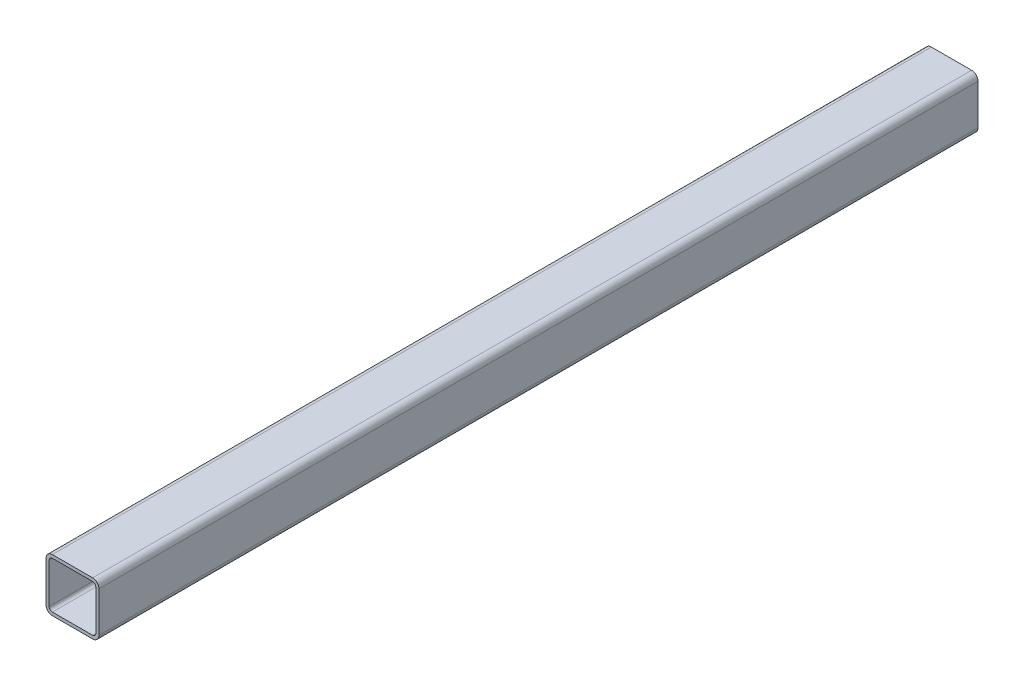
SolidWorks part; units mm, degrees
material "Q235B"
ref_plane "前视基准面" through (0, 0, 0) normal (0, 0, 1) x (1, 0, 0)
ref_plane "上视基准面" through (0, 0, 0) normal (0, 1, 0) x (1, 0, 0)
ref_plane "右视基准面" through (0, 0, 0) normal (1, 0, 0) x (0, 0, -1)
other "Configuration Table"
sketch "草图1" plane through (0, 0, 0) normal (1, 0, 0) x (0, 0, -1)
  line L0 (-415, 0) -> (415, 0)
other "Gb／6728-1986方形空心型钢 050 X 50 X 3(1)"
ref_plane "基准面1" through (0, 0, 415) normal (0, 0, -1) x (0, 1, 0)
sketch "Sketch1" plane through (0, 0, 415) normal (0, 0, -1) x (0, 1, 0)
  line L0 (-19, -22) -> (19, -22)
  line L1 (-22, -19) -> (-22, 19)
  line L2 (19, 22) -> (-19, 22)
  line L3 (22, 19) -> (22, -19)
  line L4 (-19, -25) -> (19, -25)
  line L5 (-25, -19) -> (-25, 19)
  line L6 (19, 25) -> (-19, 25)
  line L7 (25, 19) -> (25, -19)
  arc A0 (25, 19) -> (19, 25) centre (19, 19) ccw
  arc A1 (19, -25) -> (25, -19) centre (19, -19) ccw
  arc A2 (-25, -19) -> (-19, -25) centre (-19, -19) ccw
  arc A3 (-19, 25) -> (-25, 19) centre (-19, 19) ccw
  arc A4 (-19, 22) -> (-22, 19) centre (-19, 19) ccw
  arc A5 (22, 19) -> (19, 22) centre (19, 19) ccw
  arc A6 (19, -22) -> (22, -19) centre (19, -19) ccw
  arc A7 (-22, -19) -> (-19, -22) centre (-19, -19) ccw
  point P0 (-25, 0)
  point P1 (25, 0)
  point P2 (0, 25)
  point P3 (0, -25)
  point P4 (0, 0)
  point P5 (-25, -25)
  point P6 (25, -25)
  point P7 (25, 25)
  point P8 (-25, 25)
  point P33 (0, 0)
  dimension "D1" = 6
  dimension "Thickness" = 3
  dimension "V_leg" = 50
equation "\"D2@草图1\"=\"D1@草图1\"/2"
